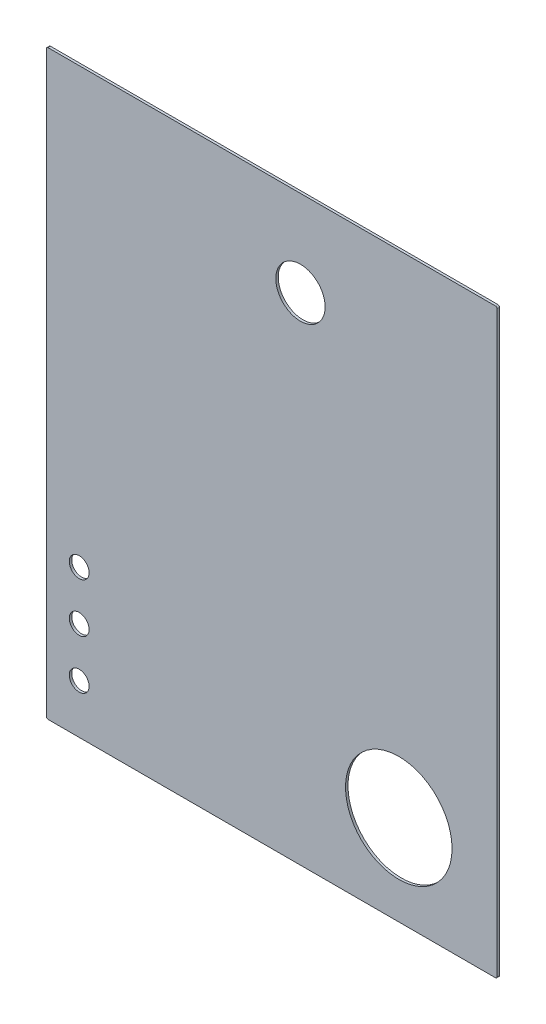
SolidWorks part; units mm, degrees
ref_plane "Front Plane" through (0, 0, 0) normal (0, 0, 1) x (1, 0, 0)
ref_plane "Top Plane" through (0, 0, 0) normal (0, 1, 0) x (1, 0, 0)
ref_plane "Right Plane" through (0, 0, 0) normal (1, 0, 0) x (0, 0, -1)
sketch "Sketch1" plane through (0, 0, 0) normal (0, 0, 1) x (1, 0, 0)
  line L0 (550, 710) -> (550, 605) construction
  line L1 (2, 0) -> (548, 0)
  line L2 (0, 2) -> (0, 708)
  line L3 (2, 710) -> (548, 710)
  line L4 (550, 2) -> (550, 708)
  line L5 (550, 605) -> (310, 605) construction
  line L6 (550, 0) -> (550, 110) construction
  line L7 (550, 110) -> (430, 110) construction
  circle A0 centre (40, 60) radius 12.1
  circle A1 centre (40, 120) radius 12.1
  circle A2 centre (40, 180) radius 12.1
  circle A3 centre (430, 110) radius 65
  circle A4 centre (40, 240) radius 12.1 [skipped]
  circle A5 centre (310, 605) radius 30.1
  arc A6 (0, 708) -> (2, 710) centre (2, 708) cw
  arc A7 (2, 0) -> (0, 2) centre (2, 2) cw
  arc A8 (548, 0) -> (550, 2) centre (548, 2) ccw
  arc A9 (548, 710) -> (550, 708) centre (548, 708) cw
  point P21 (0, 710)
  point P24 (0, 0)
  dimension "D3" = 4
  dimension "D4" = 2
  dimension "D1" = 550
  dimension "D2" = 710
extrude "Boss-Extrude1" add sketch "Sketch1" along normal blind 3
